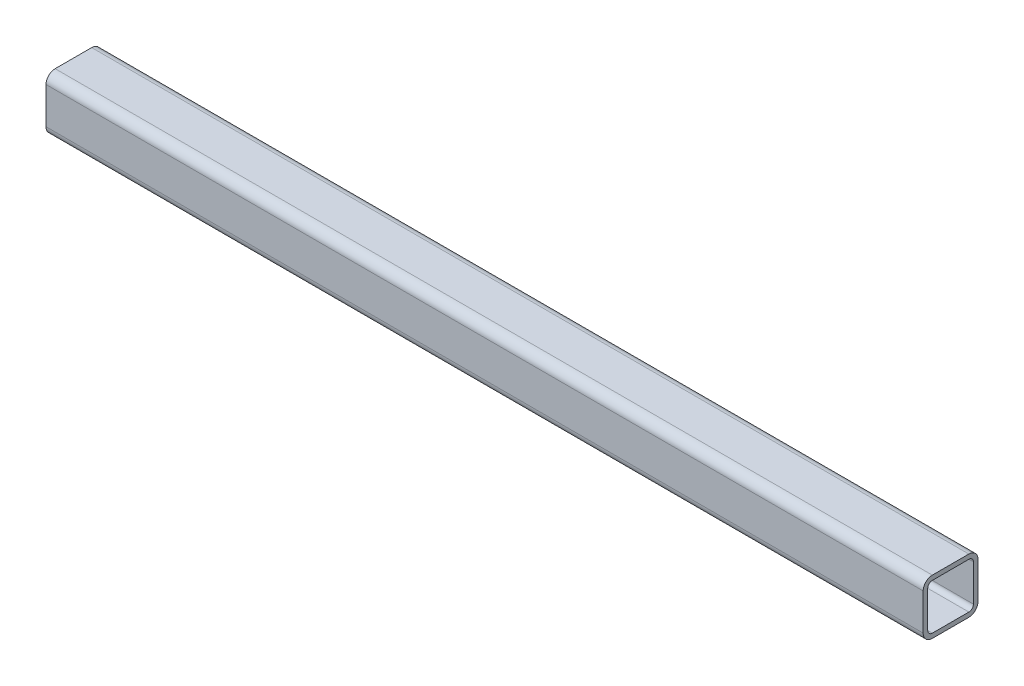
from build123d import *

# Parameters (mm, degrees)
SQUARE_TUBE_30_X_30_X_2_5_DEPTH = 480


with BuildPart() as part:
    # Sketch16 → Square tube 30 X 30 X 2.5 (new body)
    with BuildSketch(Plane.YZ.offset(-240)):
        with BuildLine():
            Line((-10, -15), (10, -15))
            ThreePointArc((10, -15), (13.535533906, -13.535533906), (15, -10))
            Line((15, -10), (15, 10))
            ThreePointArc((15, 10), (13.535533906, 13.535533906), (10, 15))
            Line((10, 15), (-10, 15))
            ThreePointArc((-10, 15), (-13.535533906, 13.535533906), (-15, 10))
            Line((-15, 10), (-15, -10))
            ThreePointArc((-15, -10), (-13.535533906, -13.535533906), (-10, -15))
        make_face()
        with BuildLine():
            Line((-10, -12.5), (10, -12.5))
            ThreePointArc((10, -12.5), (11.767766953, -11.767766953), (12.5, -10))
            Line((12.5, -10), (12.5, 10))
            ThreePointArc((12.5, 10), (11.767766953, 11.767766953), (10, 12.5))
            Line((10, 12.5), (-10, 12.5))
            ThreePointArc((-10, 12.5), (-11.767766953, 11.767766953), (-12.5, 10))
            Line((-12.5, 10), (-12.5, -10))
            ThreePointArc((-12.5, -10), (-11.767766953, -11.767766953), (-10, -12.5))
        make_face(mode=Mode.SUBTRACT)
    extrude(amount=SQUARE_TUBE_30_X_30_X_2_5_DEPTH)


solid = part.part
